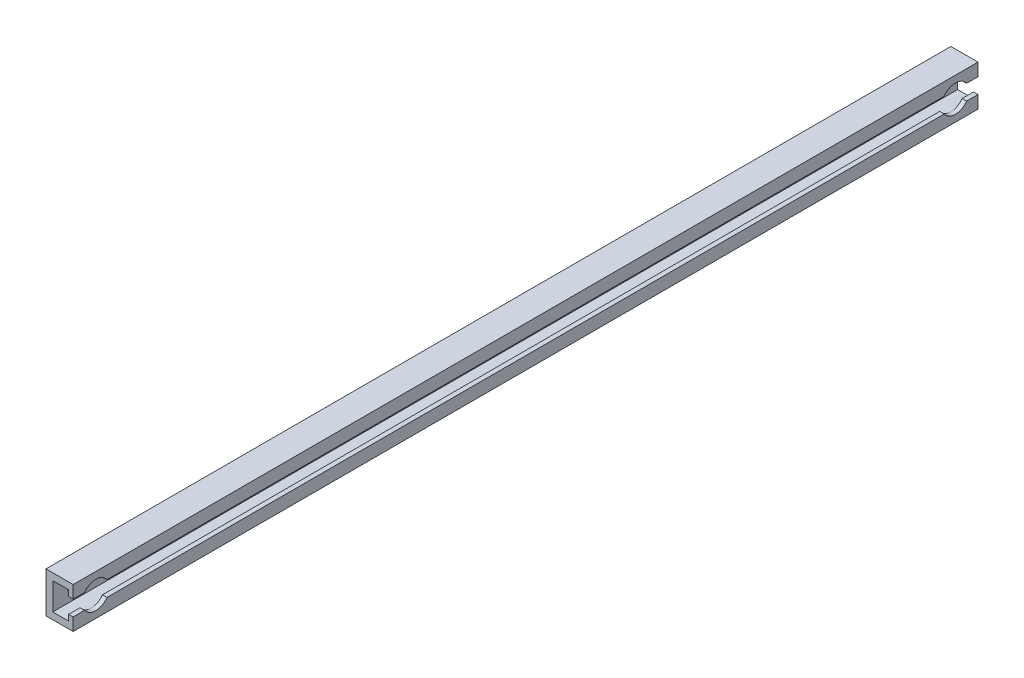
SolidWorks part; units mm, degrees
material "GY-GD-0609"
ref_plane "前视基准面" through (0, 0, 0) normal (0, 0, 1) x (1, 0, 0)
ref_plane "上视基准面" through (0, 0, 0) normal (0, 1, 0) x (1, 0, 0)
ref_plane "右视基准面" through (0, 0, 0) normal (1, 0, 0) x (0, 0, -1)
sketch "Model" plane through (0, 0, 0) normal (0, 0, 1) x (1, 0, 0)
  line L0 (235.9714, 159.9772) -> (239.4714, 159.9772)
  line L1 (235.9714, 165.9772) -> (235.9714, 159.9772)
  line L2 (239.4714, 159.9772) -> (239.4714, 161.2772)
  line L3 (239.4714, 165.9772) -> (235.9714, 165.9772)
  line L4 (239.4714, 161.2772) -> (240.4714, 161.2772)
  line L5 (239.4714, 164.6772) -> (239.4714, 165.9772)
  line L6 (240.4714, 161.2772) -> (240.4714, 158.4772)
  line L7 (240.4714, 164.6772) -> (239.4714, 164.6772)
  line L8 (240.4714, 158.4772) -> (234.4714, 158.4772)
  line L9 (240.4714, 167.4772) -> (240.4714, 164.6772)
  line L10 (234.4714, 158.4772) -> (234.4714, 167.4772)
  line L11 (234.4714, 167.4772) -> (240.4714, 167.4772)
extrude "凸台-拉伸1" add sketch "Model" along normal blind 200
sketch "草图1" plane through (234.4714, 0, 0) normal (-1, 0, 0) x (0, 0, 1)
  line L0 (0, 167.4772) -> (0, 158.4772) construction
  line L1 (200, 167.4772) -> (0, 167.4772) construction
  point P0 (0, 161.4772)
  dimension "D1" = 6
sketch "草图2" plane through (234.4714, 157.9342, -3.5511) normal (-1, 0, 0) x (0, 0, 1)
  line L0 (3.5511, 3.543) -> (4.0511, 3.543)
  line L1 (4.0511, 3.543) -> (4.5511, 3.543)
  line L2 (4.5511, 3.543) -> (5.0511, 3.543)
  line L3 (5.0511, 3.543) -> (5.5511, 3.543)
  line L4 (5.5511, 3.543) -> (6.0511, 3.543)
  line L5 (6.0511, 3.543) -> (6.5511, 3.543)
  line L6 (6.5511, 3.543) -> (7.0511, 3.543)
  line L7 (3.5511, 3.543) -> (3.5511, 3.043)
  line L8 (3.5511, 3.043) -> (3.5511, 2.543)
  line L9 (3.5511, 2.543) -> (3.5511, 2.043)
  line L10 (3.5511, 3.293) -> (4.5511, 3.293)
  line L11 (3.5511, 3.043) -> (5.0511, 3.043)
  line L12 (3.5511, 2.543) -> (6.0511, 2.543)
  line L13 (3.5511, 2.793) -> (5.5511, 2.793)
  line L14 (3.5511, 2.293) -> (6.5511, 2.293)
  line L15 (3.5511, 2.043) -> (7.0511, 2.043)
  line L16 (12.0511, 6.543) -> (12.7254, 7.2815) construction
  line L17 (12.0511, 6.543) -> (6.5511, 6.543) construction
  line L18 (12.2357, 6.3744) -> (12.8282, 6.3744)
  line L19 (12.2357, 6.3744) -> (12.0511, 6.543) construction
  line L20 (12.0511, 6.543) -> (11.4973, 7.0487) construction
  line L21 (12.0511, 6.543) -> (11.714, 6.1737) construction
  line L22 (4.5511, 3.543) -> (4.5511, 3.293)
  line L23 (5.5511, 3.543) -> (5.5511, 2.793)
  line L24 (6.5511, 6.543) -> (7.2254, 7.2815) construction
  line L25 (6.9243, 6.7007) -> (7.4224, 6.7442)
  line L26 (6.7357, 6.3744) -> (6.5511, 6.543) construction
  line L27 (6.5511, 6.543) -> (5.9973, 7.0487) construction
  line L28 (6.5511, 6.543) -> (6.214, 6.1737) construction
  line L29 (12.4148, 6.6675) -> (12.9148, 6.6675)
  line L30 (6.7357, 5.7558) -> (6.7357, 5.6479)
  line L31 (6.5755, 6.5697) -> (7.4206, 6.5697)
  line L32 (7.4206, 6.5697) -> (6.9857, 5.6479)
  line L33 (6.9857, 5.6479) -> (6.7357, 5.6479)
  line L34 (6.5755, 6.5697) -> (6.4605, 6.3478)
  line L35 (6.4605, 6.3478) -> (6.7105, 6.3478)
  line L36 (7.0511, 3.543) -> (7.5511, 3.543)
  line L37 (7.5511, 3.543) -> (8.0511, 3.543)
  line L38 (8.0511, 3.543) -> (8.5511, 3.543)
  line L39 (3.5511, 2.043) -> (3.5511, 1.543)
  line L40 (3.5511, 1.543) -> (9.0511, 1.543)
  line L41 (7.9857, 5.6479) -> (8.4857, 5.6479)
  line L42 (7.9857, 5.6479) -> (8.3278, 6.5876)
  line L43 (8.8278, 6.5876) -> (9.7357, 7.438)
  line L44 (9.7357, 7.438) -> (9.2357, 7.438)
  line L45 (9.2357, 7.438) -> (8.691, 6.9278)
  line L46 (8.691, 6.9278) -> (8.4857, 7.438)
  line L47 (8.4857, 7.438) -> (7.9857, 7.438)
  line L48 (7.9857, 7.438) -> (8.3278, 6.5876)
  line L49 (8.8278, 6.5876) -> (8.4857, 5.6479)
  line L50 (7.9857, 5.6479) -> (6.9857, 5.6479) construction
  line L51 (10.3301, 7.438) -> (9.4857, 5.6479)
  line L52 (3.5511, 1.793) -> (8.5511, 1.793)
  line L53 (8.5511, 3.543) -> (8.5511, 1.793)
  line L54 (9.4857, 5.6479) -> (10.7357, 5.6479)
  line L55 (10.7357, 5.6479) -> (10.9491, 6.1002)
  line L56 (10.9491, 6.1002) -> (10.1991, 6.1002)
  line L57 (10.1991, 6.1002) -> (10.8301, 7.438)
  line L58 (10.8301, 7.438) -> (10.3301, 7.438)
  line L59 (9.4857, 5.6479) -> (8.4857, 5.6479) construction
  line L60 (6.5511, 3.543) -> (6.5511, 2.293)
  line L61 (9.2357, 7.438) -> (8.4857, 7.438) construction
  line L62 (7.2467, 7.5806) -> (7.7406, 7.658)
  line L63 (5.3616, 5.4279) -> (5.8556, 5.5053)
  line L64 (7.1967, 7.6134) -> (6.5511, 6.543) construction
  line L65 (7.4074, 6.0265) -> (6.5511, 6.543) construction
  line L66 (6.5511, 6.543) -> (5.6473, 5.0445) construction
  line L67 (7.5511, 3.543) -> (7.5511, 1.793)
  line L68 (6.0511, 3.543) -> (6.0511, 2.543)
  line L69 (8.5511, 3.543) -> (9.0511, 3.543)
  line L70 (3.5511, 3.543) -> (3.5511, 6.543) construction
  line L71 (3.5511, 6.543) -> (6.5511, 6.543) construction
  ellipse E0 centre (12.0511, 6.543) end of major axis (11.714, 6.1737) minor radius 0.25 (12.4148, 6.6675) -> (12.2357, 6.3744) ccw
  ellipse E1 centre (12.0511, 6.543) end of major axis (11.3769, 5.8045) minor radius 0.75 (12.9148, 6.6675) -> (12.8282, 6.3744) ccw
  ellipse E2 centre (6.5511, 6.543) end of major axis (6.8883, 6.9122) minor radius 0.25 (6.9243, 6.7007) -> (6.7105, 6.3478) ccw
  ellipse E3 centre (6.5511, 6.543) end of major axis (7.2254, 7.2815) minor radius 0.75 (7.4224, 6.7442) -> (6.7357, 5.7558) ccw
  ellipse E4 centre (6.5511, 6.543) end of major axis (7.455, 8.0415) minor radius 1 (7.7406, 7.658) -> (5.6948, 7.0595) ccw
  ellipse E5 centre (6.5511, 6.543) end of major axis (7.1967, 7.6134) minor radius 1 (7.2467, 7.5806) -> (5.6948, 7.0595) ccw
  ellipse E6 centre (6.5511, 6.543) end of major axis (7.455, 8.0415) minor radius 1 (5.3616, 5.4279) -> (7.4074, 6.0265) ccw
  ellipse E7 centre (6.5511, 6.543) end of major axis (7.1967, 7.6134) minor radius 1 (5.8556, 5.5053) -> (7.4074, 6.0265) ccw
  point P107 (3.5511, 3.543)
  dimension "D1" = 0.5
  dimension "D2" = 70
  dimension "D3" = 47.602
  dimension "D4" = 11.302
  dimension "D5" = 50
  dimension "D6" = 5
  dimension "D7" = 15
extrude "切除-拉伸1" cut sketch "草图2" against normal blind 0.1 contours L29 E1 L18 E0 | L57 L58 L51 L54 L55 L56 | L49 L43 L44 L45 L46 L47 L48 L42 L41 | E5 L62 E4 | L25 E3 L30 L33 L32 L31 L34 L35 E2 | E7 L63 E6
sketch "草图3" plane through (240.4714, 0, 0) normal (1, 0, 0) x (0, 0, -1)
  line L0 (-200, 158.4772) -> (0, 158.4772) construction
  line L1 (-100, 167.4772) -> (-100, 195.2254) construction
  line L2 (-200, 167.4772) -> (0, 167.4772) construction
  circle A0 centre (-195, 162.9772) radius 3
  circle A1 centre (-5, 162.9772) radius 3
  dimension "D1" = 6
  dimension "D2" = 4.5
  dimension "D3" = 190
extrude "切除-拉伸2" cut sketch "草图3" against normal up to surface (4.5 mm away) up to face at (235.9714, 162.9772, 100)
sketch "草图4" plane through (235.9714, 0, 0) normal (1, 0, 0) x (0, 0, -1)
  circle A0 centre (-195, 162.9772) radius 1.75
  circle A1 centre (-5, 162.9772) radius 1.75
  dimension "D1" = 3.5
extrude "切除-拉伸3" cut sketch "草图4" against normal through all
